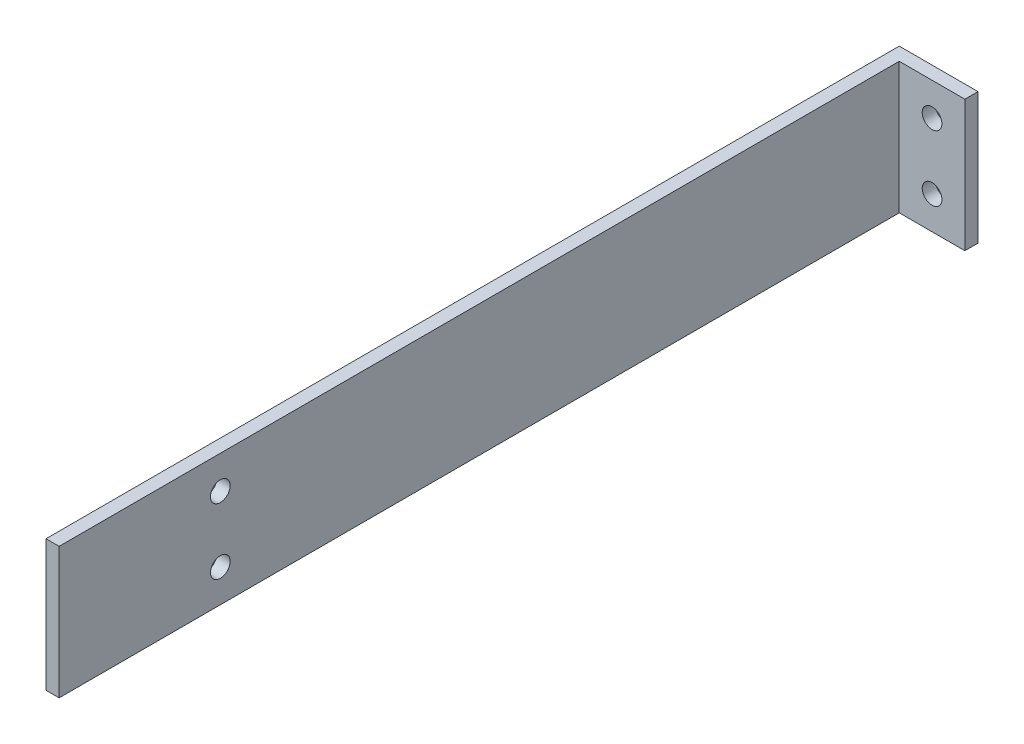
SolidWorks part; units mm, degrees
ref_plane "Front Plane" through (0, 0, 0) normal (0, 0, 1) x (1, 0, 0)
ref_plane "Top Plane" through (0, 0, 0) normal (0, 1, 0) x (1, 0, 0)
ref_plane "Right Plane" through (0, 0, 0) normal (1, 0, 0) x (0, 0, -1)
sketch "Sketch1" plane through (0, 0, 0) normal (0, 0, 1) x (1, 0, 0)
  line L0 (0, 0) -> (10, 0) construction
  line L1 (10, 10) -> (12, 10)
  line L2 (10, 10) -> (10, -10)
  line L3 (10, -10) -> (12, -10)
  line L4 (12, 10) -> (12, -10)
  line L5 (10, 10) -> (12, -10) construction
  line L6 (10, -10) -> (12, 10) construction
  point P0 (11, 0)
  dimension "D1" = 10
  dimension "D2" = 2
  dimension "D3" = 20
extrude "Boss-Extrude1" add sketch "Sketch1" along normal blind 130
sketch "Sketch2" plane through (0, 0, 0) normal (0, 0, 1) x (1, 0, 0)
  line L0 (12, -10) -> (12, 10) construction
  line L1 (12, -10) -> (12, 10)
  line L2 (12, 10) -> (22, 10)
  line L3 (22, 10) -> (22, -10)
  line L4 (22, -10) -> (12, -10)
  dimension "D1" = 10
extrude "Boss-Extrude2" add sketch "Sketch2" along normal blind 2
sketch "Sketch3" plane through (0, 0, 2) normal (0, 0, 1) x (1, 0, 0)
  line L0 (22, 0) -> (12, 0) construction
  line L1 (22, -10) -> (22, 10) construction
  line L2 (12, -10) -> (12, 10) construction
  line L3 (17, 0) -> (17, 10) construction
  line L4 (22, 10) -> (12, 10) construction
  line L5 (17, 0) -> (17, -10) construction
  circle A0 centre (17, 5) radius 1.5
  circle A1 centre (17, -5) radius 1.5
  dimension "D1" = 3
extrude "Cut-Extrude1" cut sketch "Sketch3" against normal blind 6
sketch "Sketch5" plane through (12, 0, 0) normal (1, 0, 0) x (0, 0, -1)
  line L0 (-130, 0) -> (-105.4422, 0) construction
  line L1 (-130, -10) -> (-130, 10) construction
  line L2 (-105.4422, 5) -> (-105.4422, -5) construction
  circle A0 centre (-105.4422, -5) radius 1.5
  circle A1 centre (-105.4422, 5) radius 1.5
  dimension "D2" = 3
  dimension "D1" = 10
extrude "Cut-Extrude2" cut sketch "Sketch5" against normal blind 45
